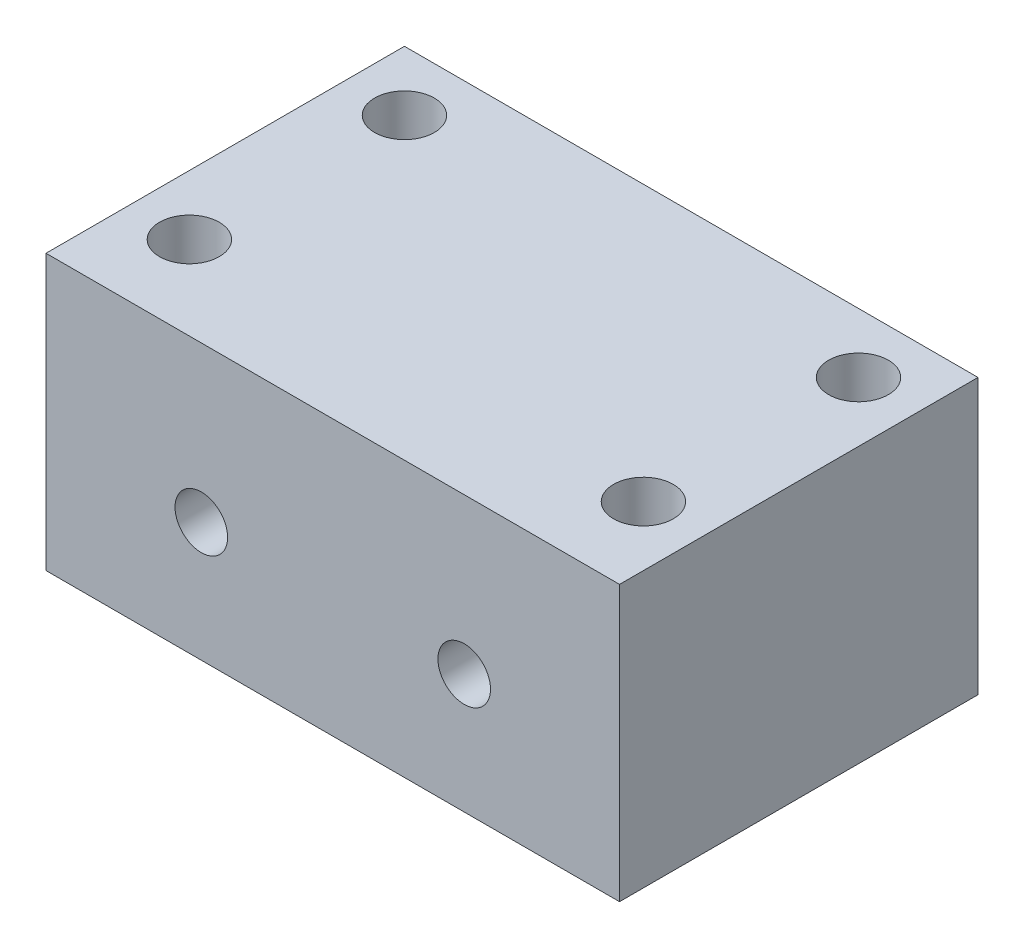
from build123d import *

# Parameters (mm, degrees)
SKETCH_1_W          = 48
SKETCH_1_H          = 30
EXTRUDE_1_DEPTH     = 30
SKETCH_2_W          = 28
SKETCH_2_H          = 15
CUT_EXTRUDE_1_DEPTH = 20
SKETCH_3_R          = 2.2
CUT_EXTRUDE_2_DEPTH = 20
SKETCH_4_R          = 2.5
CUT_EXTRUDE_3_DEPTH = 30
CUT_EXTRUDE_START   = -30
SKETCH_8_W          = 48
SKETCH_8_H          = 7
CUT_EXTRUDE_5_DEPTH = 30


with BuildPart() as part:
    # 草图1 → 凸台-拉伸1 (new body)
    with BuildSketch(Plane.XY):
        with Locations((-0.545454545, 1.527272727)):
            Rectangle(SKETCH_1_W, SKETCH_1_H)
    extrude(amount=EXTRUDE_1_DEPTH)

    # 草图2 → 切除-拉伸1 (cut)
    with BuildSketch(Plane(origin=(0, 0, 0), x_dir=(-1, 0, 0), z_dir=(0, 0, -1))):
        with Locations((0.545454545, -5.972727273)):
            Rectangle(SKETCH_2_W, SKETCH_2_H)
    extrude(amount=-CUT_EXTRUDE_1_DEPTH, mode=Mode.SUBTRACT)

    # 草图3 → 切除-拉伸2 (cut)
    with BuildSketch(Plane(origin=(0, 0, 20), x_dir=(-1, 0, 0), z_dir=(0, 0, -1))):
        with Locations((-10.454545455, -3.472727273)):
            Circle(SKETCH_3_R)
        with Locations((11.545454545, -3.472727273)):
            Circle(SKETCH_3_R)
    extrude(amount=-CUT_EXTRUDE_2_DEPTH, mode=Mode.SUBTRACT)

    # 草图4 → 切除-拉伸3 (cut)
    with BuildSketch(Plane.XZ.offset(13.472727273)):
        with Locations(Location((-19.545454545, 5, 0), (0, 0, 270))):
            Circle(SKETCH_4_R)
        with Locations(Location((-19.545454545, 23, 0), (0, 0, 270))):
            Circle(SKETCH_4_R)
        with Locations(Location((18.454545455, 23, 0), (0, 0, 270))):
            Circle(SKETCH_4_R)
        with Locations(Location((18.454545455, 5, 0), (0, 0, 270))):
            Circle(SKETCH_4_R)
    extrude(amount=-CUT_EXTRUDE_3_DEPTH, mode=Mode.SUBTRACT)

    # 草图8 → 切除-拉伸5 (cut)
    with BuildSketch(Plane.XY.offset(30).offset(CUT_EXTRUDE_START)):
        with Locations((-0.545454545, 13.027272727)):
            Rectangle(SKETCH_8_W, SKETCH_8_H)
    extrude(amount=CUT_EXTRUDE_5_DEPTH, mode=Mode.SUBTRACT)


solid = part.part
